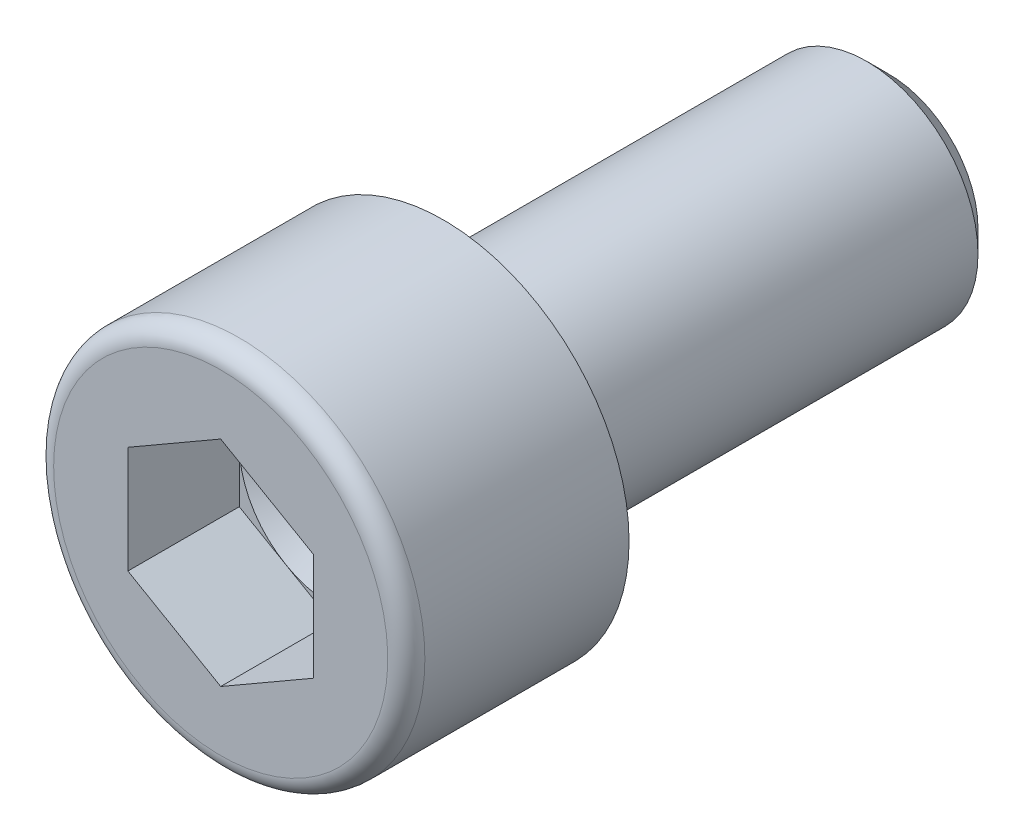
from build123d import *

# Parameters (mm, degrees)
CUT_EXTRUDE1_DEPTH = 3
FILLET1_R          = 0.5
CHAMFER1_SIZE      = 0.6
FILLET2_R          = 0.2


with BuildPart() as part:
    # Sketch3 → Revolve1 (revolve)
    with BuildSketch(Plane(origin=(0, 0, 0), x_dir=(0, 0, -1), z_dir=(1, 0, 0)), mode=Mode.PRIVATE) as revolve1_sk:
        Polygon((-6, 1), (-6, 5), (0, 5), (0, 3), (12, 3), (12, 1), align=None)
    revolve(revolve1_sk.sketch.rotate(Axis((0, 0, 6), (0, 0, -1)), 90), axis=Axis((0, 0, 6), (0, 0, -1)))

    # Sketch4 → Cut-Extrude1 (cut)
    with BuildSketch(Plane.XY.offset(6)):
        Polygon((0, 2.886751346), (-2.5, 1.443375673), (-2.5, -1.443375673), (0, -2.886751346), (2.5, -1.443375673), (2.5, 1.443375673), align=None)
    extrude(amount=-CUT_EXTRUDE1_DEPTH, mode=Mode.SUBTRACT)

    # Fillet1
    fillet1_edges = [part.edges().sort_by_distance(p)[0] for p in [
        (-5, 0, 6),
    ]]
    fillet(fillet1_edges, radius=FILLET1_R)

    # Chamfer1
    chamfer1_edges = [part.edges().sort_by_distance(p)[0] for p in [
        (-3, 0, -12),
    ]]
    chamfer(chamfer1_edges, length=CHAMFER1_SIZE)

    # Cut-Extrude2 cone 1 section (through the dimple's axis) → Cut-Extrude2 (revolve, cut)
    with BuildSketch(Plane(origin=(0, 0, 3), x_dir=(0, -1, 0), z_dir=(1, 0, 0))):
        Polygon((0, 0), (2.5, 0), (0, 1.443375673), align=None)
    revolve(axis=Axis((0, 0, 3), (0, 0, -1)), mode=Mode.SUBTRACT)

    # Fillet2
    fillet2_edges = [part.edges().sort_by_distance(p)[0] for p in [
        (-3, 0, 0),
    ]]
    fillet(fillet2_edges, radius=FILLET2_R)


solid = part.part
